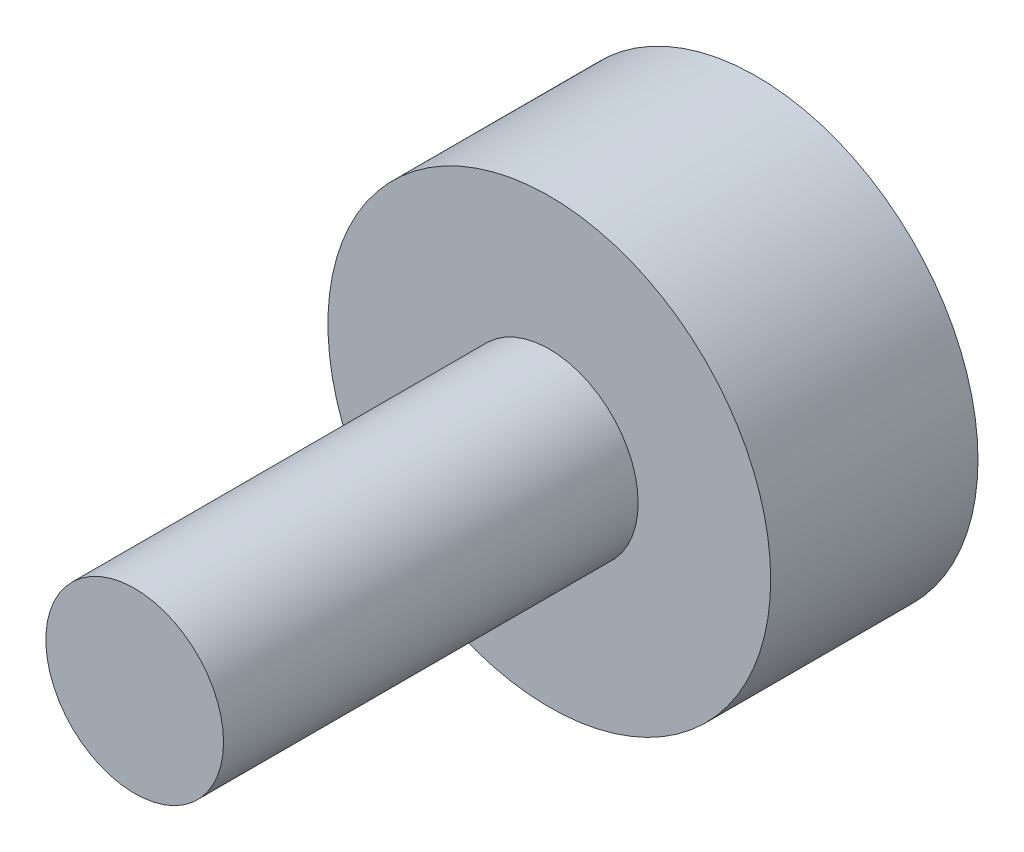
SolidWorks part; units mm, degrees
ref_plane "前视基准面" through (0, 0, 0) normal (0, 0, 1) x (1, 0, 0)
ref_plane "上视基准面" through (0, 0, 0) normal (0, 1, 0) x (1, 0, 0)
ref_plane "右视基准面" through (0, 0, 0) normal (1, 0, 0) x (0, 0, -1)
other "Configuration Table"
sketch "草图1" plane through (0, 0, 0) normal (0, 0, 1) x (1, 0, 0)
  circle A0 centre (0, 0) radius 74.75
  dimension "D1" = 149.5
extrude "凸台-拉伸1" add sketch "草图1" along normal blind 70 contours A0
sketch "草图2" plane through (0, 0, 0) normal (0, 0, -1) x (-1, 0, 0)
  circle A0 centre (0, 0) radius 16.25
  dimension "D1" = 32.5
extrude "切除-拉伸1" cut sketch "草图2" against normal blind 68 contours A0
sketch "草图3" plane through (0, 0, 70) normal (0, 0, 1) x (1, 0, 0)
  circle A0 centre (0, 0) radius 30
  dimension "D1" = 60
extrude "凸台-拉伸2" add sketch "草图3" along normal blind 140 contours A0
